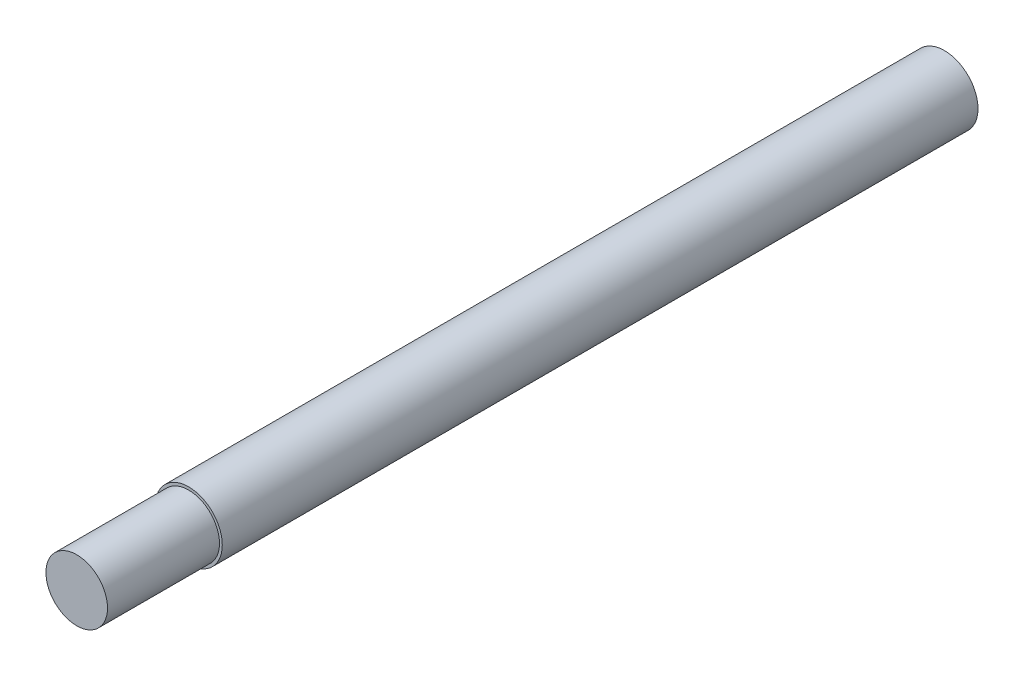
SolidWorks part; units mm, degrees
ref_plane "前视基准面" through (0, 0, 0) normal (0, 0, 1) x (1, 0, 0)
ref_plane "上视基准面" through (0, 0, 0) normal (0, 1, 0) x (1, 0, 0)
ref_plane "右视基准面" through (0, 0, 0) normal (1, 0, 0) x (0, 0, -1)
sketch "草图1" plane through (0, 0, 0) normal (0, 0, 1) x (1, 0, 0)
  circle A0 centre (0, 0) radius 6
  dimension "D1" = 12
extrude "凸台-拉伸3" add sketch "草图1" along normal mid plane 155
sketch "草图3" plane through (0, 0, 77.5) normal (0, 0, 1) x (1, 0, 0)
  circle A0 centre (0, 0) radius 5.5
  circle A1 centre (0, 0) radius 6 construction
  circle A2 centre (0, 0) radius 6
  dimension "D1" = 11
extrude "切除-拉伸1" cut sketch "草图3" against normal blind 20
